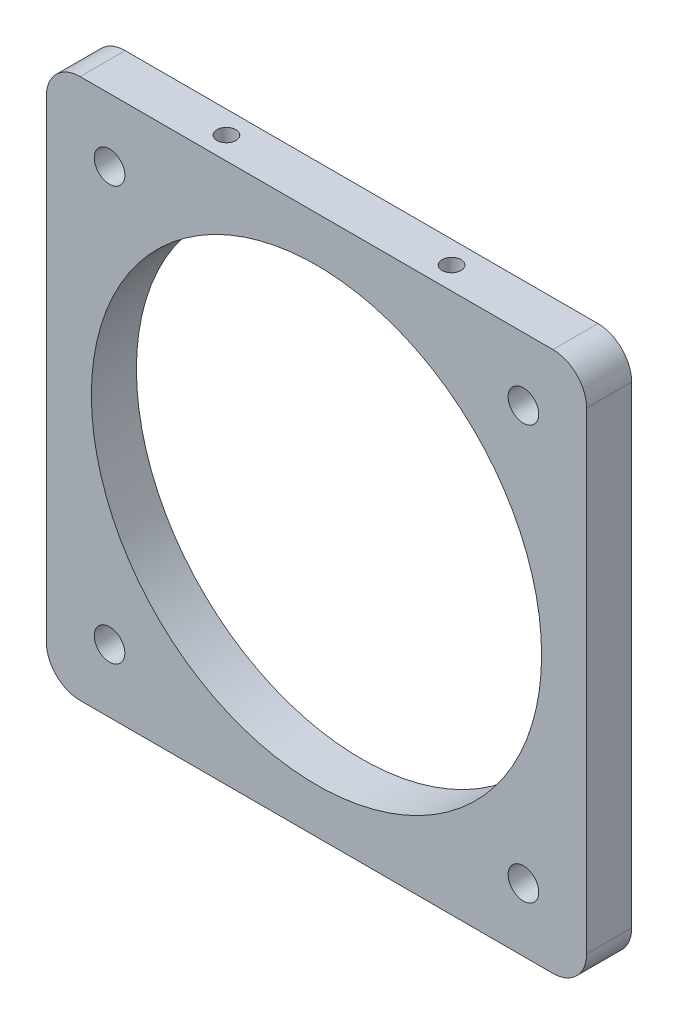
from build123d import *

# Parameters (mm, degrees)
SKETCH1_W             = 120
SKETCH1_H             = 120
BOSS_EXTRUDE1_DEPTH   = 10
FILLET1_R             = 7.5
M5_TAPPED_HOLE1_D     = 4.2
M5_TAPPED_HOLE1_DEPTH = 12.4
M5_TAPPED_HOLE1_TIP   = 1.2618073
SKETCH4_R             = 50
CUT_EXTRUDE1_DEPTH    = 10
M8_TAPPED_HOLE1_D     = 6.8
M8_TAPPED_HOLE1_DEPTH = 19.75
M8_TAPPED_HOLE1_TIP   = 2.042926105


with BuildPart() as part:
    # Sketch1 → Boss-Extrude1 (new body)
    with BuildSketch(Plane.XY):
        Rectangle(SKETCH1_W, SKETCH1_H)
    extrude(amount=BOSS_EXTRUDE1_DEPTH)

    # Fillet1
    fillet1_edges = [part.edges().sort_by_distance(p)[0] for p in [
        (-60, 60, 5),
        (60, 60, 5),
        (60, -60, 5),
        (-60, -60, 5),
    ]]
    fillet(fillet1_edges, radius=FILLET1_R)

    # M5 Tapped Hole1
    with Locations(Plane(origin=(0, 60, 0), x_dir=(1, 0, 0), z_dir=(0, 1, 0))):
        with Locations((-25, -5), (25, -5)):
            Hole(M5_TAPPED_HOLE1_D / 2, depth=M5_TAPPED_HOLE1_DEPTH)
            with Locations((0, 0, -(M5_TAPPED_HOLE1_DEPTH + M5_TAPPED_HOLE1_TIP / 2))):  # 118° drill point
                Cone(0, M5_TAPPED_HOLE1_D / 2, M5_TAPPED_HOLE1_TIP, mode=Mode.SUBTRACT)

    # Sketch4 → Cut-Extrude1 (cut)
    with BuildSketch(Plane.XY.offset(10)):
        Circle(SKETCH4_R)
    extrude(amount=-CUT_EXTRUDE1_DEPTH, mode=Mode.SUBTRACT)

    # M8 Tapped Hole1
    with Locations(Plane.XY.offset(10)):
        with Locations((-45.961940777, 45.961940777), (45.961940777, 45.961940777), (45.961940777, -45.961940777), (-45.961940777, -45.961940777)):
            Hole(M8_TAPPED_HOLE1_D / 2, depth=M8_TAPPED_HOLE1_DEPTH)
            with Locations((0, 0, -(M8_TAPPED_HOLE1_DEPTH + M8_TAPPED_HOLE1_TIP / 2))):  # 118° drill point
                Cone(0, M8_TAPPED_HOLE1_D / 2, M8_TAPPED_HOLE1_TIP, mode=Mode.SUBTRACT)


solid = part.part
